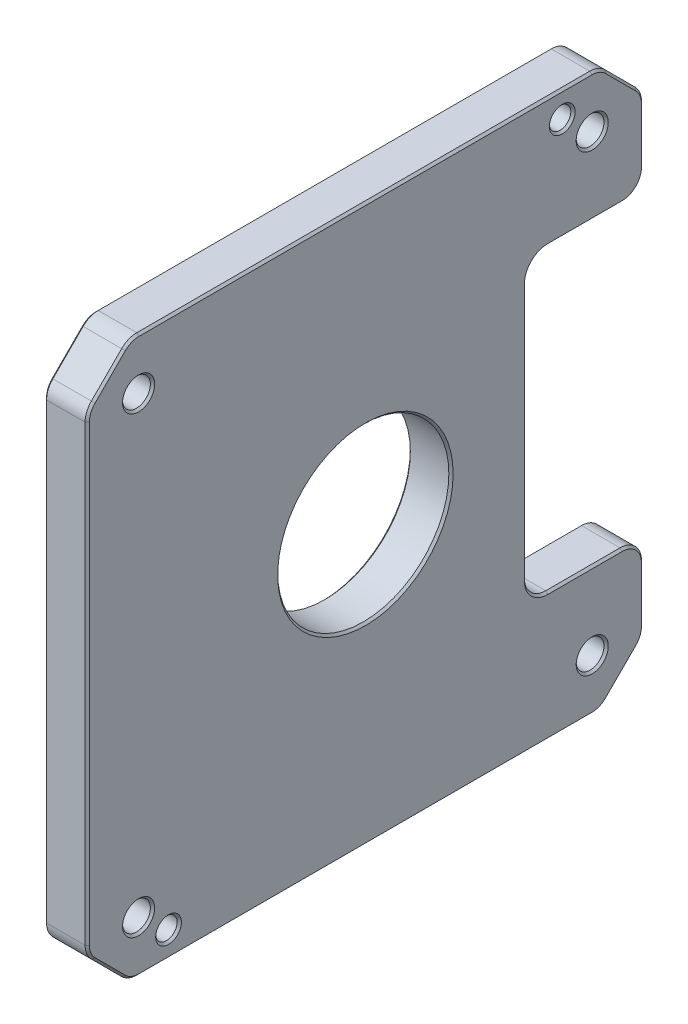
SolidWorks part; units mm, degrees
material "6061 合金"
ref_plane "前视基准面" through (0, 0, 0) normal (0, 0, 1) x (1, 0, 0)
ref_plane "上视基准面" through (0, 0, 0) normal (0, 1, 0) x (1, 0, 0)
ref_plane "右视基准面" through (0, 0, 0) normal (1, 0, 0) x (0, 0, -1)
sketch "草图1" plane through (0, 0, 0) normal (1, 0, 0) x (0, 0, -1)
  line L1 (-65, 65) -> (65, 65)
  line L2 (-65, 65) -> (-65, -65)
  line L3 (-65, -65) -> (65, -65)
  line L4 (65, 65) -> (65, -65)
  line L5 (-65, 65) -> (65, -65) construction
  line L6 (-65, -65) -> (65, 65) construction
  point P0 (0, 0)
  dimension "D1" = 130
  dimension "D2" = 130
extrude "凸台-拉伸1" add sketch "草图1" along normal blind 10
sketch "草图2" plane through (10, 0, 0) normal (1, 0, 0) x (0, 0, -1)
  line L0 (32.64, 25) -> (32.64, -25) construction
  line L1 (97.64, -35) -> (37.64, -35)
  line L2 (97.64, -35) -> (97.64, 35)
  line L3 (97.64, 35) -> (37.64, 35)
  line L4 (37.64, -35) -> (37.64, 35)
  line L5 (92.64, -25) -> (92.64, 25) construction
  line L6 (37.64, -30) -> (87.64, -30) construction
  dimension "D1" = 5
  dimension "D2" = 5
  dimension "D3" = 5
extrude "切除-拉伸1" cut sketch "草图2" against normal through all
chamfer "倒角1" distance 10 angle 45 4 edges at (5, 65, -65) (5, -65, -65) (5, 65, 65) (5, -65, 65)
sketch "草图3" plane through (10, 0, 0) normal (1, 0, 0) x (0, 0, -1)
  circle A0 centre (-53, -53) radius 3.25
  circle A1 centre (-53, 53) radius 3.25
  circle A2 centre (53, -53) radius 3.25
  circle A3 centre (53, 53) radius 3.25
extrude "切除-拉伸2" cut sketch "草图3" against normal through all
sketch "草图4" plane through (10, 0, 0) normal (1, 0, 0) x (0, 0, -1)
  circle A0 centre (-46, -59) radius 2.5
  circle A1 centre (46, 59) radius 2.5
extrude "切除-拉伸3" cut sketch "草图4" against normal through all
sketch "草图5" plane through (0, 0, 0) normal (-1, 0, 0) x (0, 0, 1)
  circle A0 centre (0, 0) radius 20
extrude "切除-拉伸6" cut sketch "草图5" against normal through all
fillet "圆角1" radius 5 2 edges at (5, -35, -37.64) (5, 35, -37.64)
fillet "圆角2" radius 5 10 edges at (5, 65, 55) (5, 55, 65) (5, -65, -55) (5, -55, -65) (5, -35, -65) (5, 35, -65) (5, 55, -65) (5, 65, -55) (5, -55, 65) (5, -65, 55)
chamfer "倒角2" distance 0.5 angle 45 62 edges at (10, 64.6194, -54.8423) (10, 60, -60) (10, 54.8423, -64.6194) (10, 46.4645, -65) (10, 36.4645, -63.5355) (10, 35, -51.32) (10, 33.5355, -39.1045) (10, 0, -37.64) (10, -33.5355, -39.1045) (10, -35, -51.32) (10, -36.4645, -63.5355) (10, -46.4645, -65) (10, -54.8423, -64.6194) (10, -60, -60) (10, -64.6194, -54.8423) (10, -65, 0) (10, -64.6194, 54.8423) (10, -60, 60) (10, -54.8423, 64.6194) (10, 0, 65) (10, 54.8423, 64.6194) (10, 60, 60) (10, 64.6194, 54.8423) (10, 65, 0) (10, -53, 49.75) (10, 53, -56.25) (10, -53, -56.25) (10, 53, 49.75) (10, -59, 43.5) (10, 59, -48.5) (10, 0, 20) (0, 54.8423, 64.6194) (0, 0, 65) (0, -54.8423, 64.6194) (0, -60, 60) (0, -64.6194, 54.8423) (0, -65, 0) (0, -64.6194, -54.8423) (0, -60, -60) (0, -54.8423, -64.6194) (0, -46.4645, -65) (0, -36.4645, -63.5355) (0, -35, -51.32) (0, -33.5355, -39.1045) (0, 0, -37.64) (0, 33.5355, -39.1045) (0, 35, -51.32) (0, 36.4645, -63.5355) (0, 46.4645, -65) (0, 54.8423, -64.6194) (0, 60, -60) (0, 64.6194, -54.8423) (0, 65, 0) (0, 64.6194, 54.8423) (0, 60, 60) (0, -53, 49.75) (0, 53, -56.25) (0, -53, -56.25) (0, 53, 49.75) (0, -59, 43.5) (0, 59, -48.5) (0, 0, 20)
